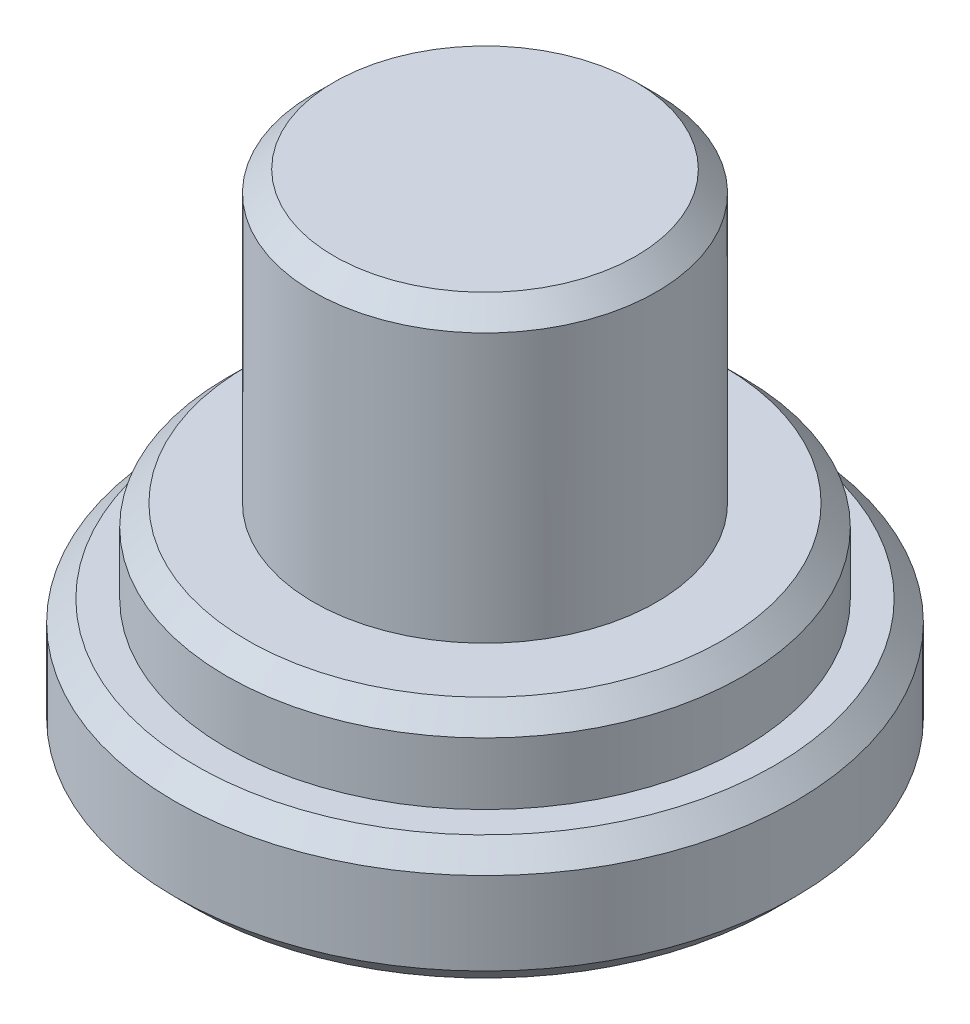
SolidWorks part; units mm, degrees
material "20#"
ref_plane "Front Plane" through (0, 0, 0) normal (0, 0, 1) x (1, 0, 0)
ref_plane "Top Plane" through (0, 0, 0) normal (0, 1, 0) x (1, 0, 0)
ref_plane "Right Plane" through (0, 0, 0) normal (1, 0, 0) x (0, 0, -1)
sketch "Sketch1" plane through (0, 0, 0) normal (0, 0, 1) x (1, 0, 0)
  line L0 (154.8784, -569.5053) -> (152.7784, -569.5053)
  line L1 (154.8784, -571.5053) -> (154.8784, -569.2053) construction
  line L2 (152.7784, -569.5053) -> (152.7784, -562.5053)
  line L3 (152.7784, -562.5053) -> (148.6284, -562.5053)
  line L4 (148.6284, -560.8053) -> (148.6284, -571.5053) construction
  line L5 (-201.3716, -571.5053) -> (163.2749, -571.5053) construction
  line L6 (156.2534, -560.8053) -> (141.0034, -560.8053) construction
  line L7 (154.8784, -569.5053) -> (154.8784, -571.5053)
  line L8 (154.8784, -571.5053) -> (156.1284, -571.5053)
  line L9 (156.1284, -571.5053) -> (156.1284, -574.5053)
  line L10 (156.1284, -574.5053) -> (148.6284, -574.5053)
  line L11 (148.6284, -562.5053) -> (148.6284, -574.5053)
  dimension "D1" = 3
  dimension "D2" = 8.3
  dimension "D3" = 2
  dimension "D4" = 15
  dimension "D5" = 12
revolve "Revolve1" add sketch "Sketch1" angle 360 about L4
chamfer "Chamfer1" distance 0.5 angle 45 4 edges at (142.3784, -569.5053, 0) (144.4784, -562.5053, 0) (141.1284, -574.5053, 0) (141.1284, -571.5053, 0)
